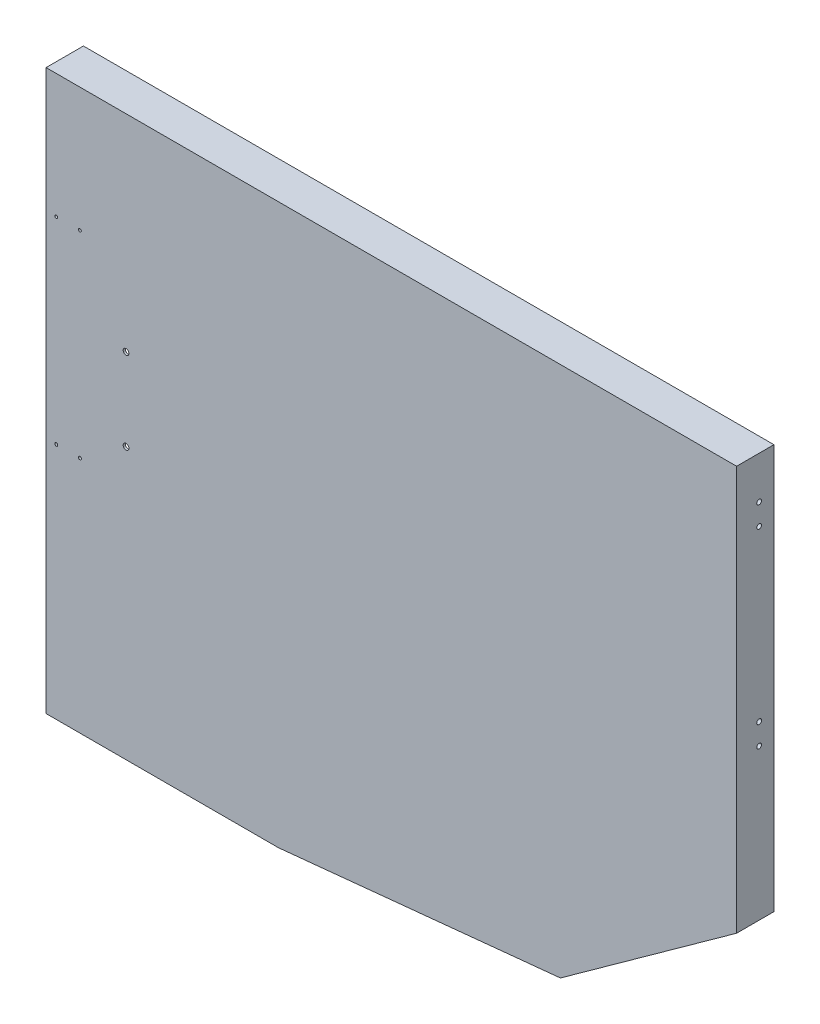
from build123d import *

# Parameters (mm, degrees)
EXTRUDE_1_DEPTH        = 53
EXTRUDE_1_2_DEPTH      = 3
EXTRUDE_2_DEPTH        = 50
EXTRUDE_3_REACH        = 966.878
CUT_EXTRUDE_1_REACH    = 695.448
SKETCH_5_R             = 4.1
HOLE_WIZARD_M8_1_D     = 6.8
HOLE_WIZARD_M8_1_DEPTH = 8
HOLE_WIZARD_M5_1_D     = 4.2
HOLE_WIZARD_M5_1_DEPTH = 14
HOLE_WIZARD_M5_1_TIP   = 1.2618073


with BuildPart() as part:
    # 草图1 → Extrude 1 (new body)
    with BuildSketch(Plane.XY):
        Polygon((-430, 375), (-111, 375), (550, 375), (550, -199), (300, -379), (-100, -419), (-430, -419), align=None)
        Polygon((-427, 372), (-111, 372), (547, 372), (547, -197.463298768), (298.9004217, -376.094995144), (-100.149626863, -416), (-427, -416), align=None, mode=Mode.SUBTRACT)
    extrude(amount=EXTRUDE_1_DEPTH)

    # 草图2 → Extrude 1 2 (add)
    with BuildSketch(Plane(origin=(0, 0, 53), x_dir=(-1, 0, 0), z_dir=(0, 0, -1))):
        Polygon((100, -419), (430, -419), (430, 375), (-550, 375), (-550, -199), (-300, -379), align=None)
    extrude(amount=EXTRUDE_1_2_DEPTH)

    # 草图3 → 凸台-拉伸2 (add)
    with BuildSketch(Plane(origin=(0, 0, 50), x_dir=(-1, 0, 0), z_dir=(0, 0, -1))):
        Polygon((-542, 375), (-550, 375), (-550, -199), (-544.865692733, -199), (-542, -201.063298768), (-542, -199.063298768), align=None)
    extrude(amount=EXTRUDE_2_DEPTH)

    # 拉伸-薄壁3: up to this plane
    extrude_3_end = Plane(origin=(280.386179605, -389.425249452, 53), z_dir=(-0.584304725845076, 0.8115343414514945, 0))
    # 草图4 → 拉伸-薄壁3 (add, up to the surface)
    with BuildSketch(Plane.XZ.offset(-372), mode=Mode.PRIVATE) as extrude_3_sk1:
        Polygon((492, 50), (542, 8), (543.286384173, 9.53140973), (493.286384173, 51.53140973), align=None)
    extrude_3_tool1 = split(extrude(extrude_3_sk1.sketch, amount=EXTRUDE_3_REACH, mode=Mode.PRIVATE), bisect_by=extrude_3_end, keep=Keep.BOTH, mode=Mode.PRIVATE)
    add(extrude_3_tool1.solids().sort_by_distance((517.643192, 372, 29.765705))[0])

    # 草图5 → 切除-拉伸1 (cut, up to next)
    with BuildSketch(Plane.XY.offset(53), mode=Mode.PRIVATE) as cut_extrude_1_sk1:
        with Locations((-316.5, 82.25)):
            Circle(SKETCH_5_R)
    cut_extrude_1_tool1 = extrude(cut_extrude_1_sk1.sketch, amount=-CUT_EXTRUDE_1_REACH, mode=Mode.PRIVATE) & part.part
    # 草图5 → 切除-拉伸1 (cut, up to next)
    with BuildSketch(Plane.XY.offset(53), mode=Mode.PRIVATE) as cut_extrude_1_sk2:
        with Locations((-316.5, -34.25)):
            Circle(SKETCH_5_R)
    cut_extrude_1_tool2 = extrude(cut_extrude_1_sk2.sketch, amount=-CUT_EXTRUDE_1_REACH, mode=Mode.PRIVATE) & part.part
    add(cut_extrude_1_tool1.solids().sort_by_distance((-316.5, 82.25, 53))[0], mode=Mode.SUBTRACT)
    add(cut_extrude_1_tool2.solids().sort_by_distance((-316.5, -34.25, 53))[0], mode=Mode.SUBTRACT)

    # M8 螺纹孔1
    with Locations(Plane(origin=(550, 0, 0), x_dir=(0, 0, -1), z_dir=(1, 0, 0))):
        with Locations((-21, 315), (-21, 285), (-21, 45), (-21, 15)):
            Hole(HOLE_WIZARD_M8_1_D / 2, depth=HOLE_WIZARD_M8_1_DEPTH)

    # M5 螺纹孔1
    with Locations(Plane.XY.offset(53)):
        with Locations((-415.514659804, 199), (-382.014659804, 199), (-415.514659804, -81), (-382.014659804, -81)):
            Hole(HOLE_WIZARD_M5_1_D / 2, depth=HOLE_WIZARD_M5_1_DEPTH)
            with Locations((0, 0, -(HOLE_WIZARD_M5_1_DEPTH + HOLE_WIZARD_M5_1_TIP / 2))):  # 118° drill point
                Cone(0, HOLE_WIZARD_M5_1_D / 2, HOLE_WIZARD_M5_1_TIP, mode=Mode.SUBTRACT)


solid = part.part
